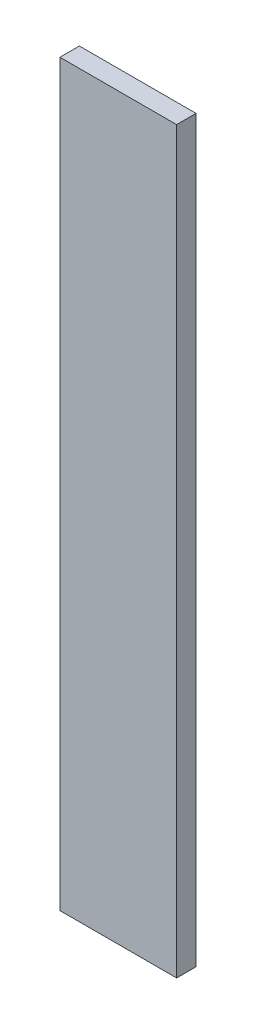
SolidWorks part; units mm, degrees
ref_plane "前视基准面" through (0, 0, 0) normal (0, 0, 1) x (1, 0, 0)
ref_plane "上视基准面" through (0, 0, 0) normal (0, 1, 0) x (1, 0, 0)
ref_plane "右视基准面" through (0, 0, 0) normal (1, 0, 0) x (0, 0, -1)
other "Configuration Table"
sketch "草图1" plane through (0, 0, 0) normal (0, 0, 1) x (1, 0, 0)
  line L1 (-30, -190) -> (30, -190)
  line L2 (-30, -190) -> (-30, 190)
  line L3 (-30, 190) -> (30, 190)
  line L4 (30, -190) -> (30, 190)
  line L5 (0, 190) -> (0, -190) construction
  line L6 (-30, 0) -> (30, 0) construction
  point P0 (0, 0)
  dimension "D1" = 60
  dimension "D2" = 380
extrude "凸台-拉伸1" add sketch "草图1" along normal blind 10
